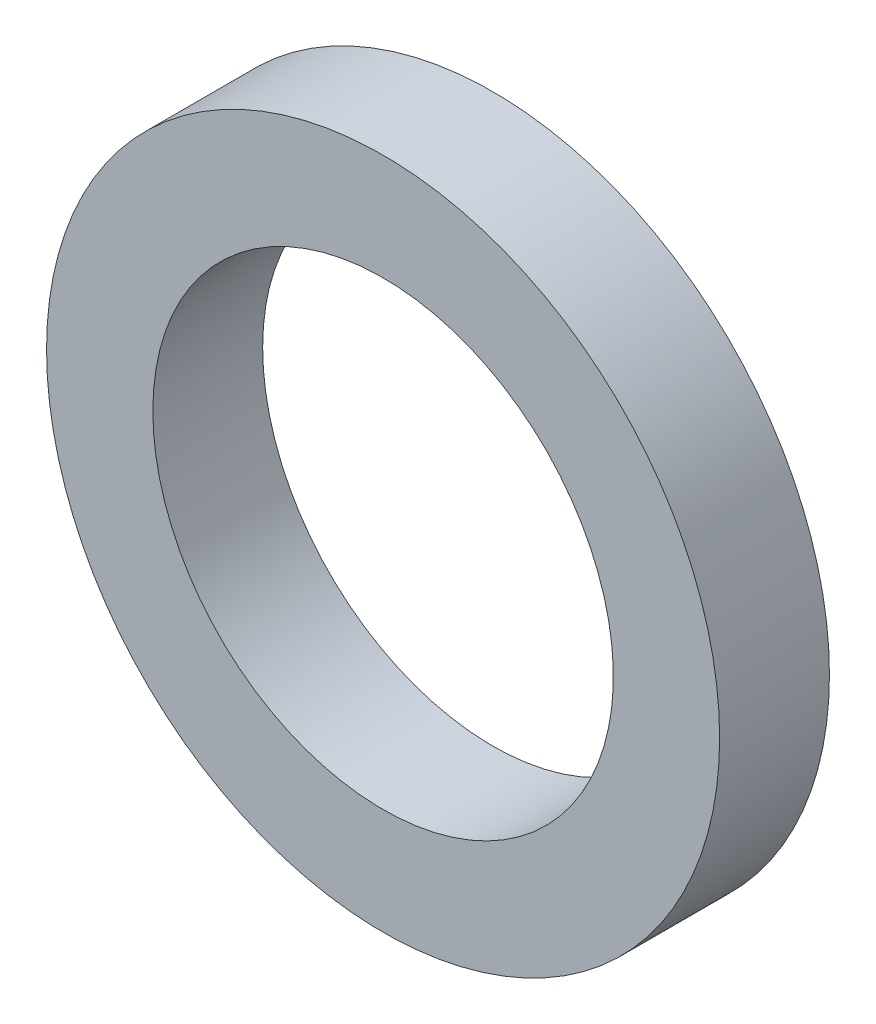
from build123d import *

# Parameters (mm, degrees)
SKETCH1_R           = 9.5
SKETCH1_R_2         = 6.5
BOSS_EXTRUDE1_DEPTH = 3.1


with BuildPart() as part:
    # Sketch1 → Boss-Extrude1 (new body)
    with BuildSketch(Plane.XY):
        with Locations(Location((0, 0, 0), (0, 0, 180))):
            Circle(SKETCH1_R)
        with Locations(Location((0, 0, 0), (0, 0, 180))):
            Circle(SKETCH1_R_2, mode=Mode.SUBTRACT)
    extrude(amount=BOSS_EXTRUDE1_DEPTH)


solid = part.part
